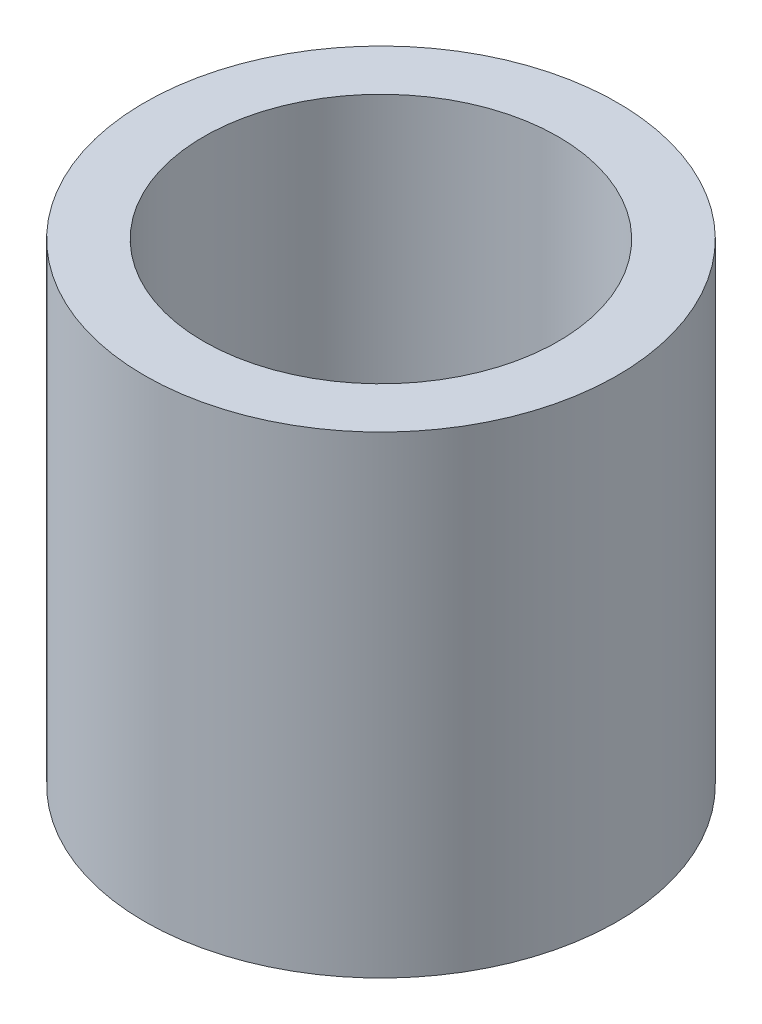
from build123d import *

# Parameters (mm, degrees)
SKETCH_1_R      = 10
SKETCH_1_R_2    = 7.5
EXTRUDE_1_DEPTH = 10


with BuildPart() as part:
    # 草图1 → 凸台-拉伸1 (new, symmetric)
    with BuildSketch(Plane(origin=(0, 0, 0), x_dir=(1, 0, 0), z_dir=(0, 1, 0))):
        with Locations(Location((0, 0, 0), (0, 0, 270))):
            Circle(SKETCH_1_R)
        with Locations(Location((0, 0, 0), (0, 0, 270))):
            Circle(SKETCH_1_R_2, mode=Mode.SUBTRACT)
    extrude(amount=EXTRUDE_1_DEPTH, both=True)


solid = part.part
